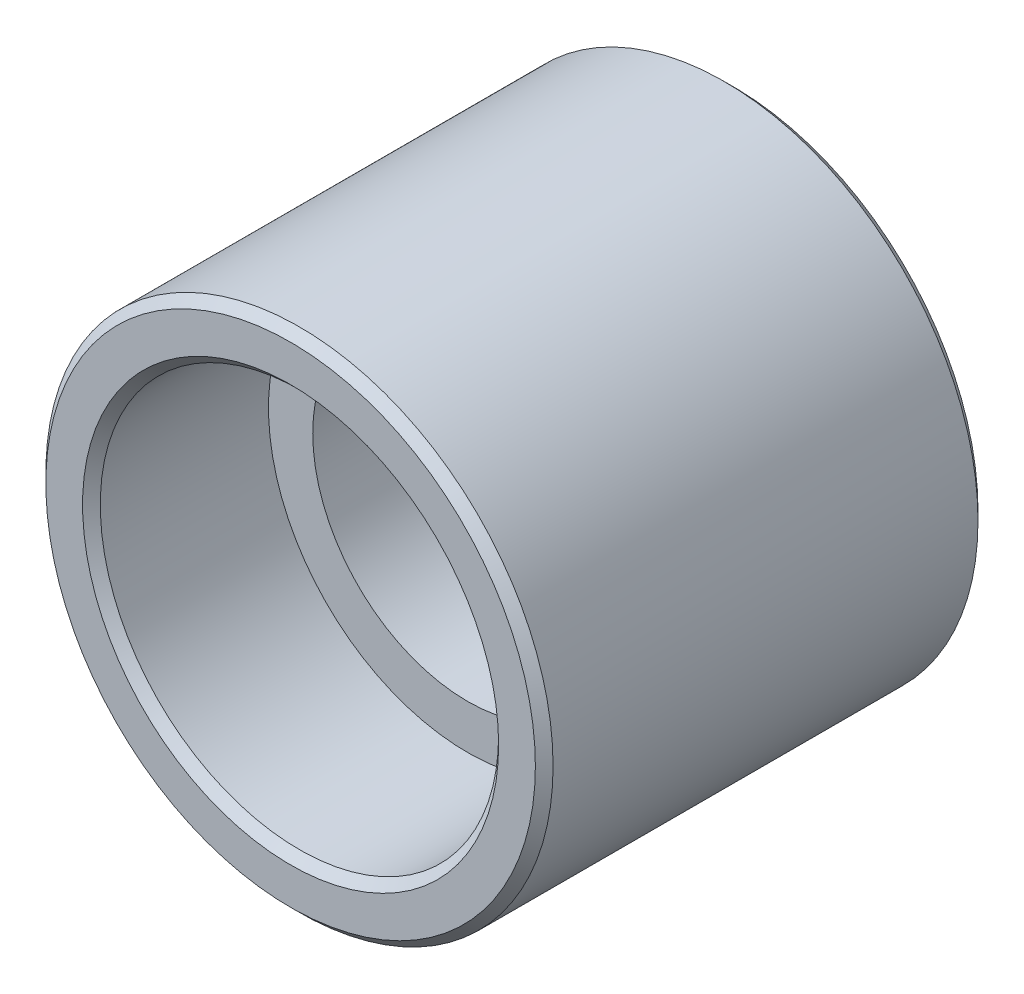
SolidWorks part; units mm, degrees
material "7075-T6"
ref_plane "Front Plane" through (0, 0, 0) normal (0, 0, 1) x (1, 0, 0)
ref_plane "Top Plane" through (0, 0, 0) normal (0, 1, 0) x (1, 0, 0)
ref_plane "Right Plane" through (0, 0, 0) normal (1, 0, 0) x (0, 0, -1)
sketch "Sketch1" plane through (0, 0, 0) normal (0, 1, 0) x (1, 0, 0)
  line L0 (4.7, 0) -> (5.53, 0)
  line L1 (5.73, 0.2) -> (5.73, 9.8)
  line L2 (5.53, 10) -> (4.7, 10)
  line L3 (4.5, 9.8) -> (4.5, 6)
  line L4 (4.5, 6) -> (3.5, 6)
  line L5 (3.5, 6) -> (3.5, 4)
  line L6 (3.5, 4) -> (4.5, 4)
  line L7 (4.5, 4) -> (4.5, 0.2)
  line L8 (0, 0) -> (0, 6.3) construction
  line L9 (4.7, 10) -> (4.5, 9.8)
  line L10 (5.73, 9.8) -> (5.53, 10)
  line L11 (5.53, 0) -> (5.73, 0.2)
  line L12 (4.5, 0.2) -> (4.7, 0)
  point P0 (4.5, 0)
  point P1 (5.73, 0)
  point P4 (5.73, 10)
  point P5 (4.5, 10)
  dimension "D1" = 11.46
  dimension "D2" = 9
  dimension "D3" = 7
  dimension "D4" = 9
  dimension "D5" = 10
  dimension "D6" = 4
  dimension "D7" = 4
revolve "Revolve1" add sketch "Sketch1" angle 360 about L8
